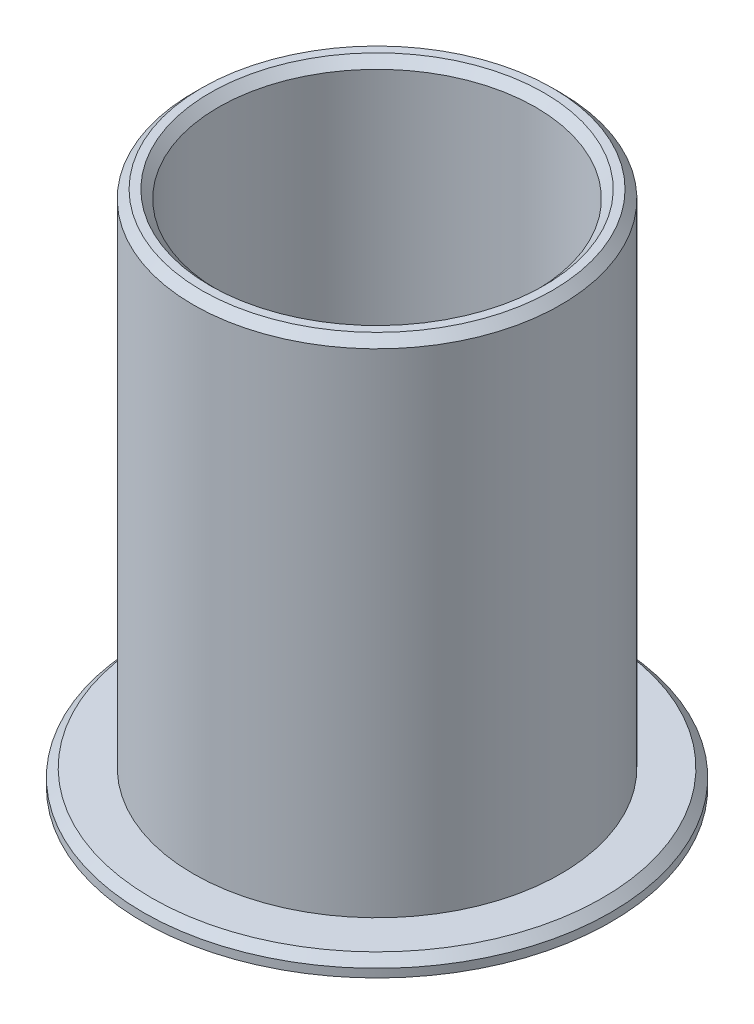
from build123d import *

# Parameters (mm, degrees)
CHAMFER1_SIZE  = 0.5
CHAMFER2_SIZE  = 1
CHAMFER2_SIZE2 = 2


with BuildPart() as part:
    # Sketch1 → Revolve1 (revolve)
    with BuildSketch(Plane.XY, mode=Mode.PRIVATE) as revolve1_sk:
        Polygon((9.5, 0), (14, 0), (14, 2), (11, 2), (11, 32), (9.5, 32), align=None)
    revolve(revolve1_sk.sketch.rotate(Axis((0, 0, 0), (0, 1, 0)), 90), axis=Axis((0, 0, 0), (0, 1, 0)))

    # Chamfer1
    chamfer1_edges = [part.edges().sort_by_distance(p)[0] for p in [
        (0, 32, 9.5),
        (0, 32, 11),
        (0, 2, 14),
        (0, 0, 9.5),
    ]]
    chamfer(chamfer1_edges, length=CHAMFER1_SIZE)

    # Chamfer2
    chamfer2_edges = [part.edges().sort_by_distance(p)[0] for p in [
        (0, 0, 14),
    ]]
    chamfer2_side = [part.faces().sort_by_distance(p)[0] for p in [
        (0, 0.75, 14),
    ]]
    chamfer(chamfer2_edges, length=CHAMFER2_SIZE, length2=CHAMFER2_SIZE2, reference=chamfer2_side[0])


solid = part.part
